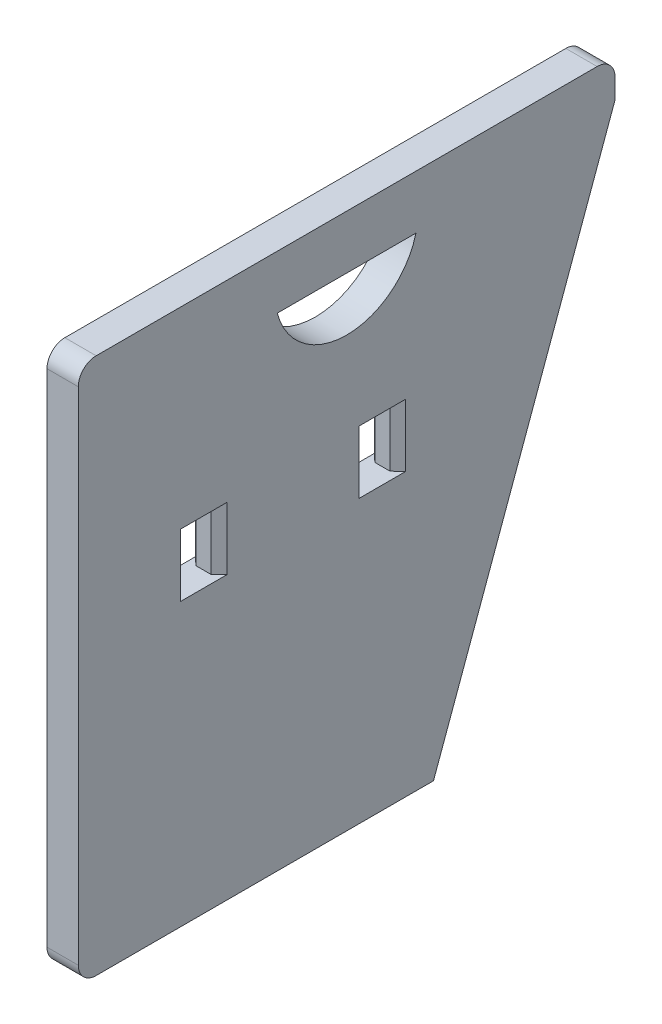
from build123d import *

# Parameters (mm, degrees)
BOSS_EXTRUDE1_DEPTH = 17.5
CUT_EXTRUDE1_START  = 50
CUT_EXTRUDE1_DEPTH  = 35
FILLET1_R           = 20
CHAMFER2_SIZE       = 15


with BuildPart() as part:
    # Sketch1 → Boss-Extrude1 (new, symmetric)
    with BuildSketch(Plane(origin=(0, 0, 0), x_dir=(0, 0, -1), z_dir=(1, 0, 0))):
        Polygon((0, 0), (0, 300), (600, 300), (600, 213.778277438), (413, -300), (0, -300), align=None)
        with BuildLine():
            Line((222.540333076, 240), (377.459666924, 240))
            ThreePointArc((377.459666924, 240), (300, 180), (222.540333076, 240))
        make_face(mode=Mode.SUBTRACT)
    extrude(amount=BOSS_EXTRUDE1_DEPTH, both=True)

    # Sketch2 → Cut-Extrude1 (cut, symmetric)
    with BuildSketch(Plane(origin=(0, 0, 0), x_dir=(1, 0, 0), z_dir=(0, 1, 0)).offset(CUT_EXTRUDE1_START)):
        Polygon((-17.5, 114), (-8.5, 122.5), (8.5, 122.5), (17.5, 114), (17.5, 166), (8.5, 157.5), (-8.5, 157.5), (-17.5, 166), align=None)
        Polygon((8.5, 357.5), (17.5, 366), (17.5, 314), (8.5, 322.5), (-8.5, 322.5), (-17.5, 314), (-17.5, 366), (-8.5, 357.5), align=None)
    extrude(amount=CUT_EXTRUDE1_DEPTH, both=True, mode=Mode.SUBTRACT)

    # Fillet1
    fillet1_edges = [part.edges().sort_by_distance(p)[0] for p in [
        (0, 300, 0),
        (0, 300, -600),
        (0, -300, 0),
    ]]
    fillet(fillet1_edges, radius=FILLET1_R)

    # Chamfer2
    chamfer2_edges = [part.edges().sort_by_distance(p)[0] for p in [
        (17.5, -43.110861281, -506.5),
    ]]
    chamfer(chamfer2_edges, length=CHAMFER2_SIZE)


solid = part.part
